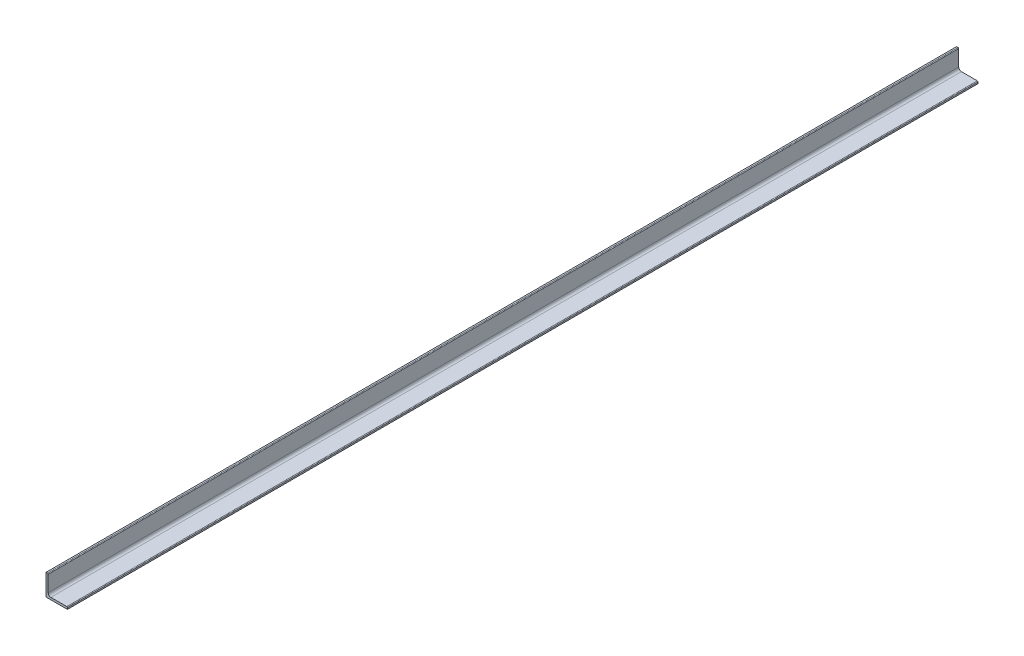
SolidWorks part; units mm, degrees
material "Q235B"
ref_plane "Plane1" through (0, 0, 0) normal (0, 0, 1) x (1, 0, 0)
ref_plane "Plane2" through (0, 0, 0) normal (0, 1, 0) x (1, 0, 0)
ref_plane "Plane3" through (0, 0, 0) normal (1, 0, 0) x (0, 0, -1)
sketch "Sketch1" plane through (0, 0, 0) normal (0, 0, 1) x (1, 0, 0)
  line L0 (0, 0) -> (0, 40)
  line L1 (0, 20) -> (4, 20) construction
  line L2 (4, 38.6667) -> (4, 9)
  line L3 (9, 4) -> (38.6667, 4)
  line L4 (20, 4) -> (20, 0) construction
  line L5 (40, 0) -> (0, 0)
  line L6 (0, 40) -> (2.6667, 40)
  line L7 (40, 0) -> (40, 2.6667)
  arc A0 (40, 2.6667) -> (38.6667, 4) centre (38.6667, 2.6667) ccw
  arc A1 (2.6667, 40) -> (4, 38.6667) centre (2.6667, 38.6667) cw
  arc A2 (9, 4) -> (4, 9) centre (9, 9) cw
  point P10 (20, 0)
  point P14 (0, 20)
  point P15 (4, 20)
  point P16 (20, 4)
  point P17 (4, 40)
  point P18 (40, 4)
  point P21 (40, 4)
  point P24 (4, 40)
extrude "Boss-Extrude1" add sketch "Sketch1" along normal blind 1700 contours L3 A0 L7 L5 L0 L6 A1 L2 A2
equation "\"D2@Sketch1\" = \"D1@Sketch1\" / 3"
